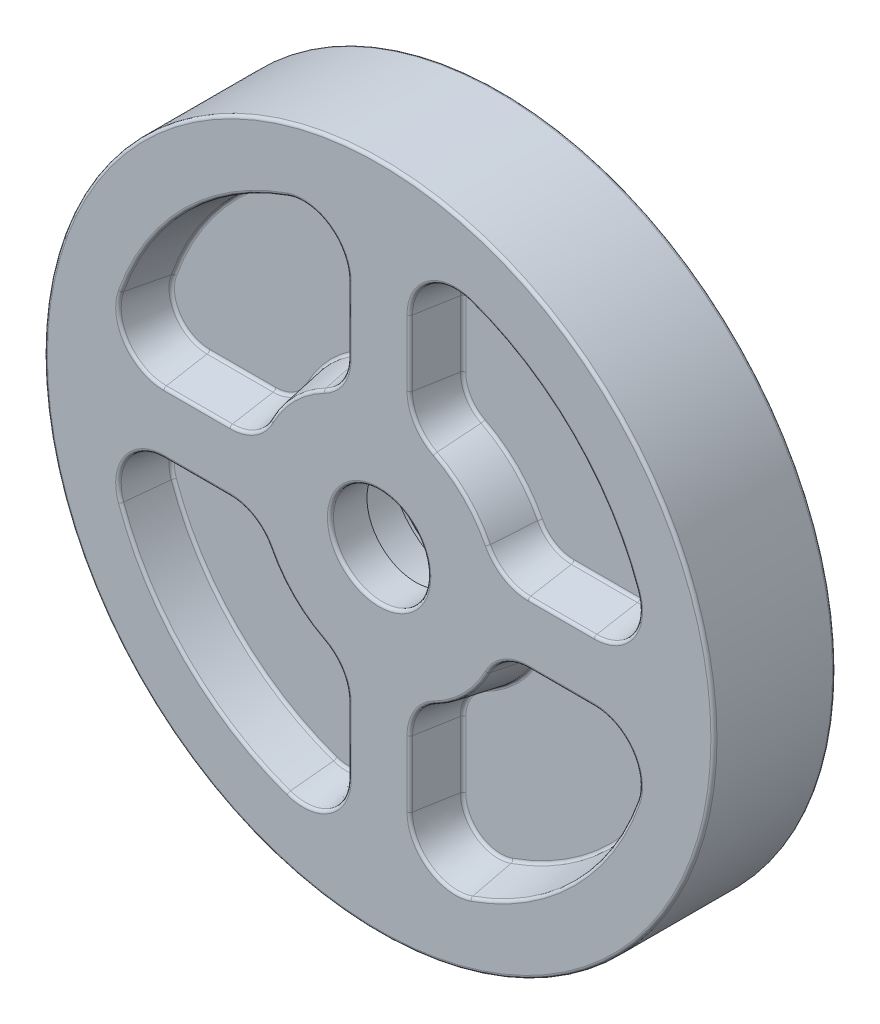
from build123d import *

# Parameters (mm, degrees)
SKETCH1_R                = 110
BOSS_EXTRUDE1_DEPTH      = 20
SKETCH2_R                = 16
CUT_EXTRUDE1_DEPTH       = 12
SKETCH3_R                = 22.5
CUT_EXTRUDE2_DEPTH       = 2
SKETCH4_R                = 26
CUT_EXTRUDE3_DEPTH       = 15
SKETCH5_R                = 27.5
CUT_EXTRUDE4_DEPTH       = 2
SKETCH6_R                = 26
CUT_EXTRUDE5_DEPTH       = 159.622192647
CUT_EXTRUDE6_DEPTH       = 15
CUT_EXTRUDE6_DRAFT       = -10
CIRPATTERN1_COPY_1_DEPTH = 15
CIRPATTERN1_COPY_1_DRAFT = -10
CIRPATTERN1_COPY_2_DEPTH = 15
CIRPATTERN1_COPY_2_DRAFT = -10
CIRPATTERN1_COPY_3_DEPTH = 15
CIRPATTERN1_COPY_3_DRAFT = -10
MIRROR1_COPY_1_DEPTH     = 15
MIRROR1_COPY_1_DRAFT     = -10
MIRROR1_COPY_2_DEPTH     = 15
MIRROR1_COPY_2_DRAFT     = -10
MIRROR1_COPY_3_DEPTH     = 15
MIRROR1_COPY_3_DRAFT     = -10
MIRROR1_COPY_4_DEPTH     = 15
MIRROR1_COPY_4_DRAFT     = -10
FILLET1_R                = 1
FILLET2_R                = 1
SKETCH8_R                = 1.5
CUT_EXTRUDE7_DEPTH       = 10


with BuildPart() as part:
    # Sketch1 → Boss-Extrude1 (new, symmetric)
    with BuildSketch(Plane.XY):
        Circle(SKETCH1_R)
    extrude(amount=BOSS_EXTRUDE1_DEPTH, both=True)

    # Sketch2 → Cut-Extrude1 (cut)
    with BuildSketch(Plane.XY.offset(20)):
        Circle(SKETCH2_R)
    extrude(amount=-CUT_EXTRUDE1_DEPTH, mode=Mode.SUBTRACT)

    # Sketch3 → Cut-Extrude2 (cut)
    with BuildSketch(Plane.XY.offset(8)):
        Circle(SKETCH3_R)
    extrude(amount=-CUT_EXTRUDE2_DEPTH, mode=Mode.SUBTRACT)

    # Sketch4 → Cut-Extrude3 (cut)
    with BuildSketch(Plane.XY.offset(6)):
        Circle(SKETCH4_R)
    extrude(amount=-CUT_EXTRUDE3_DEPTH, mode=Mode.SUBTRACT)

    # Sketch5 → Cut-Extrude4 (cut)
    with BuildSketch(Plane.XY.offset(-9)):
        Circle(SKETCH5_R)
    extrude(amount=-CUT_EXTRUDE4_DEPTH, mode=Mode.SUBTRACT)

    # Sketch6 → Cut-Extrude5 (cut, through all)
    with BuildSketch(Plane.XY.offset(-11)):
        Circle(SKETCH6_R)
    extrude(amount=-CUT_EXTRUDE5_DEPTH, mode=Mode.SUBTRACT)


with BuildPart() as cut_extrude6_tool:
    # Sketch7 → Cut-Extrude6 (with draft: the straight prism first)
    with BuildSketch(Plane(origin=(0, 0, -20), x_dir=(-1, 0, 0), z_dir=(0, 0, -1))):
        with BuildLine():
            ThreePointArc((-10, 70.710678119), (-16.339745962, 82.958126833), (-30, 84.852813742))
            ThreePointArc((-30, 84.852813742), (-63.639610307, 63.639610307), (-84.852813742, 30))
            ThreePointArc((-84.852813742, 30), (-82.958126833, 16.339745962), (-70.710678119, 10))
            Line((-70.710678119, 10), (-48.989794856, 10))
            ThreePointArc((-48.989794856, 10), (-41.156300338, 12.207957019), (-35.628941713, 18.181818182))
            ThreePointArc((-35.628941713, 18.181818182), (-28.284271247, 28.284271247), (-18.181818182, 35.628941713))
            ThreePointArc((-18.181818182, 35.628941713), (-12.207957019, 41.156300338), (-10, 48.989794856))
            Line((-10, 48.989794856), (-10, 70.710678119))
        make_face()
    extrude(amount=-CUT_EXTRUDE6_DEPTH)
    # Cut-Extrude6: the draft: its side faces are tilted about the plane it starts from
    cut_extrude6_sides = [cut_extrude6_tool.faces().sort_by_distance(p)[0] for p in [
        (12.207957019, 41.156300338, -12.5),
        (10, 59.850236487, -12.5),
        (16.339745962, 82.958126833, -12.5),
        (63.639610307, 63.639610307, -12.5),
        (82.958126833, 16.339745962, -12.5),
        (59.850236487, 10, -12.5),
        (41.156300338, 12.207957019, -12.5),
        (28.284271247, 28.284271247, -12.5),
    ]]
    draft(cut_extrude6_sides, Plane(origin=(0, 0, -20), x_dir=(-1, 0, 0), z_dir=(0, 0, -1)), CUT_EXTRUDE6_DRAFT)


with BuildPart() as part_1:
    add(part.part)

    # Cut-Extrude6: cut by cut_extrude6_tool
    add(cut_extrude6_tool.part, mode=Mode.SUBTRACT)


with BuildPart() as cirpattern1_copy_1_tool:
    # CirPattern1 copy 1 sketch → CirPattern1 copy 1 (with draft: the straight prism first)
    with BuildSketch(Plane(origin=(0, 0, -20), x_dir=(0, -1, 0), z_dir=(0, 0, -1))):
        with BuildLine():
            ThreePointArc((-10, 70.710678119), (-16.339745962, 82.958126833), (-30, 84.852813742))
            ThreePointArc((-30, 84.852813742), (-63.639610307, 63.639610307), (-84.852813742, 30))
            ThreePointArc((-84.852813742, 30), (-82.958126833, 16.339745962), (-70.710678119, 10))
            Line((-70.710678119, 10), (-48.989794856, 10))
            ThreePointArc((-48.989794856, 10), (-41.156300338, 12.207957019), (-35.628941713, 18.181818182))
            ThreePointArc((-35.628941713, 18.181818182), (-28.284271247, 28.284271247), (-18.181818182, 35.628941713))
            ThreePointArc((-18.181818182, 35.628941713), (-12.207957019, 41.156300338), (-10, 48.989794856))
            Line((-10, 48.989794856), (-10, 70.710678119))
        make_face()
    extrude(amount=-CIRPATTERN1_COPY_1_DEPTH)
    # CirPattern1 copy 1: the draft: its side faces are tilted about the plane it starts from
    cirpattern1_copy_1_sides = [cirpattern1_copy_1_tool.faces().sort_by_distance(p)[0] for p in [
        (-41.156300338, 12.207957019, -12.5),
        (-59.850236487, 10, -12.5),
        (-82.958126833, 16.339745962, -12.5),
        (-63.639610307, 63.639610307, -12.5),
        (-16.339745962, 82.958126833, -12.5),
        (-10, 59.850236487, -12.5),
        (-12.207957019, 41.156300338, -12.5),
        (-28.284271247, 28.284271247, -12.5),
    ]]
    draft(cirpattern1_copy_1_sides, Plane(origin=(0, 0, -20), x_dir=(0, -1, 0), z_dir=(0, 0, -1)), CIRPATTERN1_COPY_1_DRAFT)


with BuildPart() as part_2:
    add(part_1.part)

    # CirPattern1 copy 1: cut by cirpattern1_copy_1_tool
    add(cirpattern1_copy_1_tool.part, mode=Mode.SUBTRACT)


with BuildPart() as cirpattern1_copy_2_tool:
    # CirPattern1 copy 2 sketch → CirPattern1 copy 2 (with draft: the straight prism first)
    with BuildSketch(Plane(origin=(0, 0, -20), x_dir=(1, 0, 0), z_dir=(0, 0, -1))):
        with BuildLine():
            ThreePointArc((-10, 70.710678119), (-16.339745962, 82.958126833), (-30, 84.852813742))
            ThreePointArc((-30, 84.852813742), (-63.639610307, 63.639610307), (-84.852813742, 30))
            ThreePointArc((-84.852813742, 30), (-82.958126833, 16.339745962), (-70.710678119, 10))
            Line((-70.710678119, 10), (-48.989794856, 10))
            ThreePointArc((-48.989794856, 10), (-41.156300338, 12.207957019), (-35.628941713, 18.181818182))
            ThreePointArc((-35.628941713, 18.181818182), (-28.284271247, 28.284271247), (-18.181818182, 35.628941713))
            ThreePointArc((-18.181818182, 35.628941713), (-12.207957019, 41.156300338), (-10, 48.989794856))
            Line((-10, 48.989794856), (-10, 70.710678119))
        make_face()
    extrude(amount=-CIRPATTERN1_COPY_2_DEPTH)
    # CirPattern1 copy 2: the draft: its side faces are tilted about the plane it starts from
    cirpattern1_copy_2_sides = [cirpattern1_copy_2_tool.faces().sort_by_distance(p)[0] for p in [
        (-12.207957019, -41.156300338, -12.5),
        (-10, -59.850236487, -12.5),
        (-16.339745962, -82.958126833, -12.5),
        (-63.639610307, -63.639610307, -12.5),
        (-82.958126833, -16.339745962, -12.5),
        (-59.850236487, -10, -12.5),
        (-41.156300338, -12.207957019, -12.5),
        (-28.284271247, -28.284271247, -12.5),
    ]]
    draft(cirpattern1_copy_2_sides, Plane(origin=(0, 0, -20), x_dir=(1, 0, 0), z_dir=(0, 0, -1)), CIRPATTERN1_COPY_2_DRAFT)


with BuildPart() as part_3:
    add(part_2.part)

    # CirPattern1 copy 2: cut by cirpattern1_copy_2_tool
    add(cirpattern1_copy_2_tool.part, mode=Mode.SUBTRACT)


with BuildPart() as cirpattern1_copy_3_tool:
    # CirPattern1 copy 3 sketch → CirPattern1 copy 3 (with draft: the straight prism first)
    with BuildSketch(Plane.YX.offset(20)):
        with BuildLine():
            ThreePointArc((-10, 70.710678119), (-16.339745962, 82.958126833), (-30, 84.852813742))
            ThreePointArc((-30, 84.852813742), (-63.639610307, 63.639610307), (-84.852813742, 30))
            ThreePointArc((-84.852813742, 30), (-82.958126833, 16.339745962), (-70.710678119, 10))
            Line((-70.710678119, 10), (-48.989794856, 10))
            ThreePointArc((-48.989794856, 10), (-41.156300338, 12.207957019), (-35.628941713, 18.181818182))
            ThreePointArc((-35.628941713, 18.181818182), (-28.284271247, 28.284271247), (-18.181818182, 35.628941713))
            ThreePointArc((-18.181818182, 35.628941713), (-12.207957019, 41.156300338), (-10, 48.989794856))
            Line((-10, 48.989794856), (-10, 70.710678119))
        make_face()
    extrude(amount=-CIRPATTERN1_COPY_3_DEPTH)
    # CirPattern1 copy 3: the draft: its side faces are tilted about the plane it starts from
    cirpattern1_copy_3_sides = [cirpattern1_copy_3_tool.faces().sort_by_distance(p)[0] for p in [
        (41.156300338, -12.207957019, -12.5),
        (59.850236487, -10, -12.5),
        (82.958126833, -16.339745962, -12.5),
        (63.639610307, -63.639610307, -12.5),
        (16.339745962, -82.958126833, -12.5),
        (10, -59.850236487, -12.5),
        (12.207957019, -41.156300338, -12.5),
        (28.284271247, -28.284271247, -12.5),
    ]]
    draft(cirpattern1_copy_3_sides, Plane.YX.offset(20), CIRPATTERN1_COPY_3_DRAFT)


with BuildPart() as part_4:
    add(part_3.part)

    # CirPattern1 copy 3: cut by cirpattern1_copy_3_tool
    add(cirpattern1_copy_3_tool.part, mode=Mode.SUBTRACT)


with BuildPart() as mirror1_copy_1_tool:
    # Mirror1 copy 1 sketch → Mirror1 copy 1 (with draft: the straight prism first)
    with BuildSketch(Plane(origin=(0, 0, 20), x_dir=(-1, 0, 0), z_dir=(0, 0, 1))):
        with BuildLine():
            ThreePointArc((-10, -70.710678119), (-16.339745962, -82.958126833), (-30, -84.852813742))
            ThreePointArc((-30, -84.852813742), (-63.639610307, -63.639610307), (-84.852813742, -30))
            ThreePointArc((-84.852813742, -30), (-82.958126833, -16.339745962), (-70.710678119, -10))
            Line((-70.710678119, -10), (-48.989794856, -10))
            ThreePointArc((-48.989794856, -10), (-41.156300338, -12.207957019), (-35.628941713, -18.181818182))
            ThreePointArc((-35.628941713, -18.181818182), (-28.284271247, -28.284271247), (-18.181818182, -35.628941713))
            ThreePointArc((-18.181818182, -35.628941713), (-12.207957019, -41.156300338), (-10, -48.989794856))
            Line((-10, -48.989794856), (-10, -70.710678119))
        make_face()
    extrude(amount=-MIRROR1_COPY_1_DEPTH)
    # Mirror1 copy 1: the draft: its side faces are tilted about the plane it starts from
    mirror1_copy_1_sides = [mirror1_copy_1_tool.faces().sort_by_distance(p)[0] for p in [
        (12.207957019, 41.156300338, 12.5),
        (10, 59.850236487, 12.5),
        (16.339745962, 82.958126833, 12.5),
        (63.639610307, 63.639610307, 12.5),
        (82.958126833, 16.339745962, 12.5),
        (59.850236487, 10, 12.5),
        (41.156300338, 12.207957019, 12.5),
        (28.284271247, 28.284271247, 12.5),
    ]]
    draft(mirror1_copy_1_sides, Plane(origin=(0, 0, 20), x_dir=(-1, 0, 0), z_dir=(0, 0, 1)), MIRROR1_COPY_1_DRAFT)


with BuildPart() as part_5:
    add(part_4.part)

    # Mirror1 copy 1: cut by mirror1_copy_1_tool
    add(mirror1_copy_1_tool.part, mode=Mode.SUBTRACT)


with BuildPart() as mirror1_copy_2_tool:
    # Mirror1 copy 2 sketch → Mirror1 copy 2 (with draft: the straight prism first)
    with BuildSketch(Plane(origin=(0, 0, 20), x_dir=(0, -1, 0), z_dir=(0, 0, 1))):
        with BuildLine():
            ThreePointArc((-10, -70.710678119), (-16.339745962, -82.958126833), (-30, -84.852813742))
            ThreePointArc((-30, -84.852813742), (-63.639610307, -63.639610307), (-84.852813742, -30))
            ThreePointArc((-84.852813742, -30), (-82.958126833, -16.339745962), (-70.710678119, -10))
            Line((-70.710678119, -10), (-48.989794856, -10))
            ThreePointArc((-48.989794856, -10), (-41.156300338, -12.207957019), (-35.628941713, -18.181818182))
            ThreePointArc((-35.628941713, -18.181818182), (-28.284271247, -28.284271247), (-18.181818182, -35.628941713))
            ThreePointArc((-18.181818182, -35.628941713), (-12.207957019, -41.156300338), (-10, -48.989794856))
            Line((-10, -48.989794856), (-10, -70.710678119))
        make_face()
    extrude(amount=-MIRROR1_COPY_2_DEPTH)
    # Mirror1 copy 2: the draft: its side faces are tilted about the plane it starts from
    mirror1_copy_2_sides = [mirror1_copy_2_tool.faces().sort_by_distance(p)[0] for p in [
        (-41.156300338, 12.207957019, 12.5),
        (-59.850236487, 10, 12.5),
        (-82.958126833, 16.339745962, 12.5),
        (-63.639610307, 63.639610307, 12.5),
        (-16.339745962, 82.958126833, 12.5),
        (-10, 59.850236487, 12.5),
        (-12.207957019, 41.156300338, 12.5),
        (-28.284271247, 28.284271247, 12.5),
    ]]
    draft(mirror1_copy_2_sides, Plane(origin=(0, 0, 20), x_dir=(0, -1, 0), z_dir=(0, 0, 1)), MIRROR1_COPY_2_DRAFT)


with BuildPart() as part_6:
    add(part_5.part)

    # Mirror1 copy 2: cut by mirror1_copy_2_tool
    add(mirror1_copy_2_tool.part, mode=Mode.SUBTRACT)


with BuildPart() as mirror1_copy_3_tool:
    # Mirror1 copy 3 sketch → Mirror1 copy 3 (with draft: the straight prism first)
    with BuildSketch(Plane.XY.offset(20)):
        with BuildLine():
            ThreePointArc((-10, -70.710678119), (-16.339745962, -82.958126833), (-30, -84.852813742))
            ThreePointArc((-30, -84.852813742), (-63.639610307, -63.639610307), (-84.852813742, -30))
            ThreePointArc((-84.852813742, -30), (-82.958126833, -16.339745962), (-70.710678119, -10))
            Line((-70.710678119, -10), (-48.989794856, -10))
            ThreePointArc((-48.989794856, -10), (-41.156300338, -12.207957019), (-35.628941713, -18.181818182))
            ThreePointArc((-35.628941713, -18.181818182), (-28.284271247, -28.284271247), (-18.181818182, -35.628941713))
            ThreePointArc((-18.181818182, -35.628941713), (-12.207957019, -41.156300338), (-10, -48.989794856))
            Line((-10, -48.989794856), (-10, -70.710678119))
        make_face()
    extrude(amount=-MIRROR1_COPY_3_DEPTH)
    # Mirror1 copy 3: the draft: its side faces are tilted about the plane it starts from
    mirror1_copy_3_sides = [mirror1_copy_3_tool.faces().sort_by_distance(p)[0] for p in [
        (-12.207957019, -41.156300338, 12.5),
        (-10, -59.850236487, 12.5),
        (-16.339745962, -82.958126833, 12.5),
        (-63.639610307, -63.639610307, 12.5),
        (-82.958126833, -16.339745962, 12.5),
        (-59.850236487, -10, 12.5),
        (-41.156300338, -12.207957019, 12.5),
        (-28.284271247, -28.284271247, 12.5),
    ]]
    draft(mirror1_copy_3_sides, Plane.XY.offset(20), MIRROR1_COPY_3_DRAFT)


with BuildPart() as part_7:
    add(part_6.part)

    # Mirror1 copy 3: cut by mirror1_copy_3_tool
    add(mirror1_copy_3_tool.part, mode=Mode.SUBTRACT)


with BuildPart() as mirror1_copy_4_tool:
    # Mirror1 copy 4 sketch → Mirror1 copy 4 (with draft: the straight prism first)
    with BuildSketch(Plane(origin=(0, 0, 20), x_dir=(0, 1, 0), z_dir=(0, 0, 1))):
        with BuildLine():
            ThreePointArc((-10, -70.710678119), (-16.339745962, -82.958126833), (-30, -84.852813742))
            ThreePointArc((-30, -84.852813742), (-63.639610307, -63.639610307), (-84.852813742, -30))
            ThreePointArc((-84.852813742, -30), (-82.958126833, -16.339745962), (-70.710678119, -10))
            Line((-70.710678119, -10), (-48.989794856, -10))
            ThreePointArc((-48.989794856, -10), (-41.156300338, -12.207957019), (-35.628941713, -18.181818182))
            ThreePointArc((-35.628941713, -18.181818182), (-28.284271247, -28.284271247), (-18.181818182, -35.628941713))
            ThreePointArc((-18.181818182, -35.628941713), (-12.207957019, -41.156300338), (-10, -48.989794856))
            Line((-10, -48.989794856), (-10, -70.710678119))
        make_face()
    extrude(amount=-MIRROR1_COPY_4_DEPTH)
    # Mirror1 copy 4: the draft: its side faces are tilted about the plane it starts from
    mirror1_copy_4_sides = [mirror1_copy_4_tool.faces().sort_by_distance(p)[0] for p in [
        (41.156300338, -12.207957019, 12.5),
        (59.850236487, -10, 12.5),
        (82.958126833, -16.339745962, 12.5),
        (63.639610307, -63.639610307, 12.5),
        (16.339745962, -82.958126833, 12.5),
        (10, -59.850236487, 12.5),
        (12.207957019, -41.156300338, 12.5),
        (28.284271247, -28.284271247, 12.5),
    ]]
    draft(mirror1_copy_4_sides, Plane(origin=(0, 0, 20), x_dir=(0, 1, 0), z_dir=(0, 0, 1)), MIRROR1_COPY_4_DRAFT)


with BuildPart() as part_8:
    add(part_7.part)

    # Mirror1 copy 4: cut by mirror1_copy_4_tool
    add(mirror1_copy_4_tool.part, mode=Mode.SUBTRACT)

    # Fillet1
    fillet1_edges = [part_8.edges().sort_by_distance(p)[0] for p in [
        (-110, 0, -20),
        (-26, 0, -20),
        (42.537556774, 14.463539335, -5),
        (59.850236487, 12.644904711, -5),
        (80.798571179, 17.866782409, -5),
        (61.76938025, 61.76938025, -5),
        (17.866782409, 80.798571179, -5),
        (12.644904711, 59.850236487, -5),
        (14.463539335, 42.537556774, -5),
        (30.154501304, 30.154501304, -5),
        (41.156300338, 12.207957019, -20),
        (28.284271247, 28.284271247, -20),
        (12.207957019, 41.156300338, -20),
        (10, 59.850236487, -20),
        (16.339745962, 82.958126833, -20),
        (63.639610307, 63.639610307, -20),
        (82.958126833, 16.339745962, -20),
        (59.850236487, 10, -20),
        (14.463539335, -42.537556774, -5),
        (12.644904711, -59.850236487, -5),
        (17.866782409, -80.798571179, -5),
        (61.76938025, -61.76938025, -5),
        (80.798571179, -17.866782409, -5),
        (59.850236487, -12.644904711, -5),
        (42.537556774, -14.463539335, -5),
        (30.154501304, -30.154501304, -5),
        (12.207957019, -41.156300338, -20),
        (28.284271247, -28.284271247, -20),
        (41.156300338, -12.207957019, -20),
        (59.850236487, -10, -20),
        (82.958126833, -16.339745962, -20),
        (63.639610307, -63.639610307, -20),
        (16.339745962, -82.958126833, -20),
        (10, -59.850236487, -20),
        (-42.537556774, -14.463539335, -5),
        (-59.850236487, -12.644904711, -5),
        (-80.798571179, -17.866782409, -5),
        (-61.76938025, -61.76938025, -5),
        (-17.866782409, -80.798571179, -5),
        (-12.644904711, -59.850236487, -5),
        (-14.463539335, -42.537556774, -5),
        (-30.154501304, -30.154501304, -5),
        (-41.156300338, -12.207957019, -20),
        (-28.284271247, -28.284271247, -20),
        (-12.207957019, -41.156300338, -20),
        (-10, -59.850236487, -20),
        (-16.339745962, -82.958126833, -20),
        (-63.639610307, -63.639610307, -20),
        (-82.958126833, -16.339745962, -20),
        (-59.850236487, -10, -20),
        (-14.463539335, 42.537556774, -5),
        (-12.644904711, 59.850236487, -5),
        (-17.866782409, 80.798571179, -5),
        (-61.76938025, 61.76938025, -5),
        (-80.798571179, 17.866782409, -5),
        (-59.850236487, 12.644904711, -5),
        (-42.537556774, 14.463539335, -5),
        (-30.154501304, 30.154501304, -5),
        (-12.207957019, 41.156300338, -20),
        (-28.284271247, 28.284271247, -20),
        (-41.156300338, 12.207957019, -20),
        (-59.850236487, 10, -20),
        (-82.958126833, 16.339745962, -20),
        (-63.639610307, 63.639610307, -20),
        (-16.339745962, 82.958126833, -20),
        (-10, 59.850236487, -20),
    ]]
    fillet(fillet1_edges, radius=FILLET1_R)

    # Fillet2
    fillet2_edges = [part_8.edges().sort_by_distance(p)[0] for p in [
        (41.156300338, 12.207957019, 20),
        (28.284271247, 28.284271247, 20),
        (12.207957019, 41.156300338, 20),
        (10, 59.850236487, 20),
        (16.339745962, 82.958126833, 20),
        (63.639610307, 63.639610307, 20),
        (82.958126833, 16.339745962, 20),
        (59.850236487, 10, 20),
        (42.537556774, 14.463539335, 5),
        (30.154501304, 30.154501304, 5),
        (14.463539335, 42.537556774, 5),
        (12.644904711, 59.850236487, 5),
        (17.866782409, 80.798571179, 5),
        (61.76938025, 61.76938025, 5),
        (80.798571179, 17.866782409, 5),
        (59.850236487, 12.644904711, 5),
        (12.207957019, -41.156300338, 20),
        (28.284271247, -28.284271247, 20),
        (41.156300338, -12.207957019, 20),
        (59.850236487, -10, 20),
        (82.958126833, -16.339745962, 20),
        (63.639610307, -63.639610307, 20),
        (16.339745962, -82.958126833, 20),
        (10, -59.850236487, 20),
        (14.463539335, -42.537556774, 5),
        (30.154501304, -30.154501304, 5),
        (42.537556774, -14.463539335, 5),
        (59.850236487, -12.644904711, 5),
        (80.798571179, -17.866782409, 5),
        (61.76938025, -61.76938025, 5),
        (17.866782409, -80.798571179, 5),
        (12.644904711, -59.850236487, 5),
        (-41.156300338, -12.207957019, 20),
        (-28.284271247, -28.284271247, 20),
        (-12.207957019, -41.156300338, 20),
        (-10, -59.850236487, 20),
        (-16.339745962, -82.958126833, 20),
        (-63.639610307, -63.639610307, 20),
        (-82.958126833, -16.339745962, 20),
        (-59.850236487, -10, 20),
        (-42.537556774, -14.463539335, 5),
        (-30.154501304, -30.154501304, 5),
        (-14.463539335, -42.537556774, 5),
        (-12.644904711, -59.850236487, 5),
        (-17.866782409, -80.798571179, 5),
        (-61.76938025, -61.76938025, 5),
        (-80.798571179, -17.866782409, 5),
        (-59.850236487, -12.644904711, 5),
        (-12.207957019, 41.156300338, 20),
        (-28.284271247, 28.284271247, 20),
        (-41.156300338, 12.207957019, 20),
        (-59.850236487, 10, 20),
        (-82.958126833, 16.339745962, 20),
        (-63.639610307, 63.639610307, 20),
        (-16.339745962, 82.958126833, 20),
        (-10, 59.850236487, 20),
        (-14.463539335, 42.537556774, 5),
        (-30.154501304, 30.154501304, 5),
        (-42.537556774, 14.463539335, 5),
        (-59.850236487, 12.644904711, 5),
        (-80.798571179, 17.866782409, 5),
        (-61.76938025, 61.76938025, 5),
        (-17.866782409, 80.798571179, 5),
        (-12.644904711, 59.850236487, 5),
        (-110, 0, 20),
        (-16, 0, 20),
    ]]
    fillet(fillet2_edges, radius=FILLET2_R)

    # Sketch8 → Cut-Extrude7 (cut)
    with BuildSketch(Plane(origin=(0, 0, -20), x_dir=(-1, 0, 0), z_dir=(0, 0, -1))):
        with Locations((0, 32.5)):
            Circle(SKETCH8_R)
        with Locations((28.145825623, -16.25)):
            Circle(SKETCH8_R)
        with Locations((-28.145825623, -16.25)):
            Circle(SKETCH8_R)
    extrude(amount=-CUT_EXTRUDE7_DEPTH, mode=Mode.SUBTRACT)


solid = part_8.part
